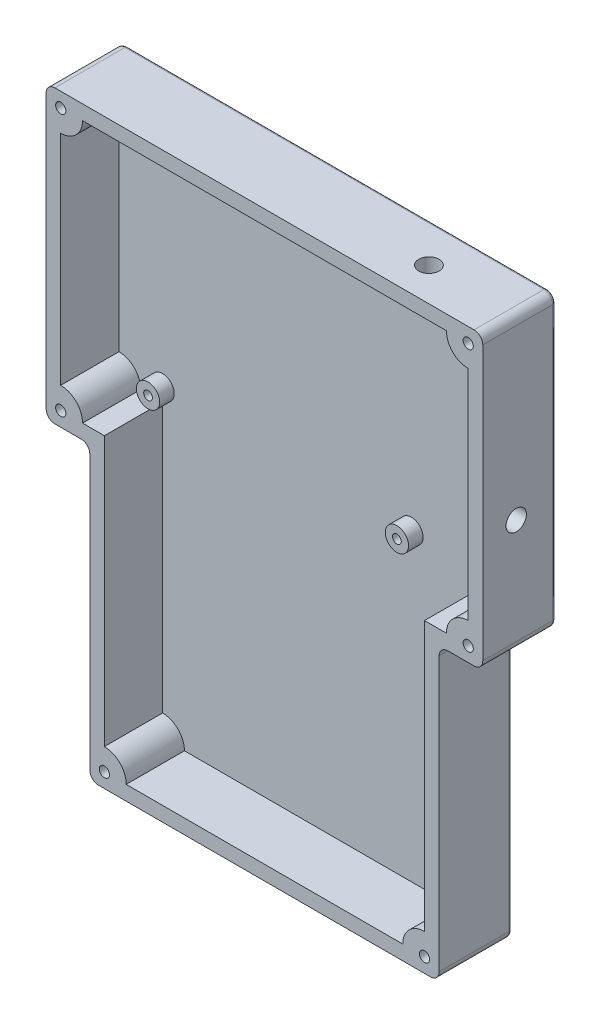
SolidWorks part; units mm, degrees
ref_plane "Front Plane" through (0, 0, 0) normal (0, 0, 1) x (1, 0, 0)
ref_plane "Top Plane" through (0, 0, 0) normal (0, 1, 0) x (1, 0, 0)
ref_plane "Right Plane" through (0, 0, 0) normal (1, 0, 0) x (0, 0, -1)
other "Configuration Table"
sketch "Sketch1" plane through (0, 0, 0) normal (0, 0, 1) x (1, 0, 0)
  line L0 (0, 0) -> (0, 200) construction
  line L1 (75, 200) -> (-75, 200)
  line L2 (-75, 200) -> (-75, 100)
  line L3 (-75, 100) -> (-60, 100)
  line L4 (-60, 100) -> (-60, 0)
  line L5 (-60, 0) -> (60, 0)
  line L6 (60, 100) -> (60, 0)
  line L7 (75, 100) -> (60, 100)
  line L8 (75, 200) -> (75, 100)
  point P11 (0, 151)
  dimension "D1" = 150
  dimension "D2" = 200
  dimension "D3" = 100
  dimension "D4" = 120
extrude "Boss-Extrude1" add sketch "Sketch1" along normal blind 25
sketch "Sketch2" plane through (0, 0, 25) normal (0, 0, 1) x (1, 0, 0)
  line L0 (70, 105) -> (70, 195)
  line L1 (70, 195) -> (-70, 195)
  line L2 (-70, 195) -> (-70, 105)
  line L3 (-70, 105) -> (-55, 105)
  line L4 (-55, 105) -> (-55, 5)
  line L5 (-55, 5) -> (55, 5)
  line L6 (55, 5) -> (55, 105)
  line L7 (55, 105) -> (70, 105)
extrude "Cut-Extrude1" cut sketch "Sketch2" against normal blind 20
fillet "Fillet1" radius 3 8 edges at (60, 100, 12.5) (-60, 100, 12.5) (-60, 0, 12.5) (60, 0, 12.5) (75, 100, 12.5) (75, 200, 12.5) (-75, 100, 12.5) (-75, 200, 12.5)
fillet "Fillet2" radius 1 16 edges at (74.1213, 100.8787, 0) (67.5, 100, 0) (60.8787, 99.1213, 0) (60, 50, 0) (59.1213, 0.8787, 0) (0, 0, 0) (-59.1213, 0.8787, 0) (-60, 50, 0) (-60.8787, 99.1213, 0) (-67.5, 100, 0) (-74.1213, 100.8787, 0) (-75, 150, 0) (-74.1213, 199.1213, 0) (0, 200, 0) (74.1213, 199.1213, 0) (75, 150, 0)
sketch "Sketch5" plane through (0, 0, 5) normal (0, 0, 1) x (1, 0, 0)
  line L3 (30.5, 109.5) -> (-55, 109.5) construction
  line L4 (30.5, 109.5) -> (30.5, 190.5) construction
  line L5 (30.5, 190.5) -> (-55, 190.5) construction
  line L6 (-55, 109.5) -> (-55, 190.5) construction
  line L7 (30.5, 109.5) -> (-55, 190.5) construction
  line L8 (30.5, 190.5) -> (-55, 109.5) construction
  line L9 (-75, 197) -> (-75, 103) construction
  line L10 (72, 200) -> (-72, 200) construction
  circle A0 centre (-55, 190.5) radius 4
  circle A1 centre (-55, 190.5) radius 1.5
  circle A2 centre (30.5, 190.5) radius 4
  circle A3 centre (30.5, 190.5) radius 1.5
  circle A4 centre (-55, 109.5) radius 4
  circle A5 centre (-55, 109.5) radius 1.5
  circle A6 centre (30.5, 109.5) radius 4
  circle A7 centre (30.5, 109.5) radius 1.5
  point P5 (-12.25, 150)
  dimension "D4" = 8
  dimension "D5" = 3
  dimension "D6" = 8
  dimension "D7" = 3
  dimension "D8" = 8
  dimension "D9" = 3
  dimension "D10" = 8
  dimension "D11" = 3
  dimension "D12" = 20
  dimension "D1" = 85.5
  dimension "D2" = 81
  dimension "D3" = 50
extrude "Boss-Extrude2" add sketch "Sketch5" along normal blind 5
sketch "Sketch6" plane through (0, 0, 25) normal (0, 0, 1) x (1, 0, 0)
  line L7 (-71.7471, 196.7489) -> (-62.7068, 196.7489)
  line L13 (-71.7471, 196.7489) -> (-71.7471, 187.7063)
  line L20 (71.5003, 195.7716) -> (62.5398, 195.7716)
  line L21 (71.5003, 195.7716) -> (71.5003, 187.6516)
  line L24 (71.5003, 103.14) -> (62.7343, 103.14)
  line L25 (71.5003, 103.14) -> (71.5003, 112.3484)
  line L28 (-56.4248, 4.34) -> (-47.5291, 4.34)
  line L29 (-56.4248, 4.34) -> (-56.4248, 12.3634)
  line L32 (56.3159, 4.34) -> (47.5291, 4.34)
  line L33 (56.3159, 4.34) -> (56.3159, 12.3837)
  line L36 (-71.7471, 102.6318) -> (-62.8837, 102.6318)
  line L37 (-71.7471, 102.6318) -> (-71.7471, 112.2937)
  arc A0 (62.5398, 195.7716) -> (71.5003, 187.6516) centre (70, 195) ccw
  arc A1 (71.5003, 112.3484) -> (62.7343, 103.14) centre (70, 105) ccw
  arc A2 (56.3159, 12.3837) -> (47.5291, 4.34) centre (55, 5) ccw
  arc A3 (-47.5291, 4.34) -> (-56.4248, 12.3634) centre (-55, 5) ccw
  arc A4 (-62.8837, 102.6318) -> (-71.7471, 112.2937) centre (-70, 105) ccw
  arc A5 (-71.7471, 187.7063) -> (-62.7068, 196.7489) centre (-70, 195) ccw
  dimension "D1" = 15
extrude "Boss-Extrude3" add sketch "Sketch6" against normal blind 25
sketch "Sketch7" plane through (0, 0, 25) normal (0, 0, 1) x (1, 0, 0)
  line L0 (0, 195) -> (0, 102.4209) construction
  line L1 (62.5, 195) -> (-62.5, 195) construction
  circle A0 centre (-70, 195) radius 1.75
  circle A1 centre (-70, 105) radius 1.75
  circle A2 centre (-55, 5) radius 1.75
  circle A3 centre (55, 5) radius 1.75
  circle A4 centre (70, 105) radius 1.75
  circle A5 centre (70, 195) radius 1.75
  dimension "D1" = 3.5
extrude "Cut-Extrude4" cut sketch "Sketch7" against normal blind 20
sketch "Sketch8" plane through (0, 0, 0) normal (0, 0, -1) x (-1, 0, 0)
  line L0 (0, 199) -> (0, -6.9096) construction
  line L1 (72, 199) -> (-72, 199) construction
  circle A0 centre (-70, 195) radius 3.75
  circle A1 centre (-70, 105) radius 3.75
  circle A2 centre (-55, 5) radius 3.75
  circle A3 centre (55, 5) radius 3.75
  circle A4 centre (70, 105) radius 3.75
  circle A5 centre (70, 195) radius 3.75
  dimension "D1" = 7.5
extrude "Cut-Extrude5" cut sketch "Sketch8" against normal blind 8
sketch "Sketch9" plane through (75, 0, 0) normal (1, 0, 0) x (0, 0, -1)
  line L0 (0, 197) -> (0, 103) construction
  line L1 (-25, 200) -> (-1, 200) construction
  circle A0 centre (-13.5, 139.14) radius 3.5
  dimension "D1" = 7
  dimension "D2" = 13.5
  dimension "D3" = 60.86
extrude "Cut-Extrude6" cut sketch "Sketch9" against normal up to next
sketch "Sketch10" plane through (0, 200, 0) normal (0, 1, 0) x (1, 0, 0)
  line L0 (-72, 0) -> (72, 0) construction
  line L1 (75, -1) -> (75, -25) construction
  circle A0 centre (45, -13.5) radius 3.5
  dimension "D1" = 7
  dimension "D2" = 13.5
  dimension "D3" = 30
extrude "Cut-Extrude7" cut sketch "Sketch10" against normal up to next
